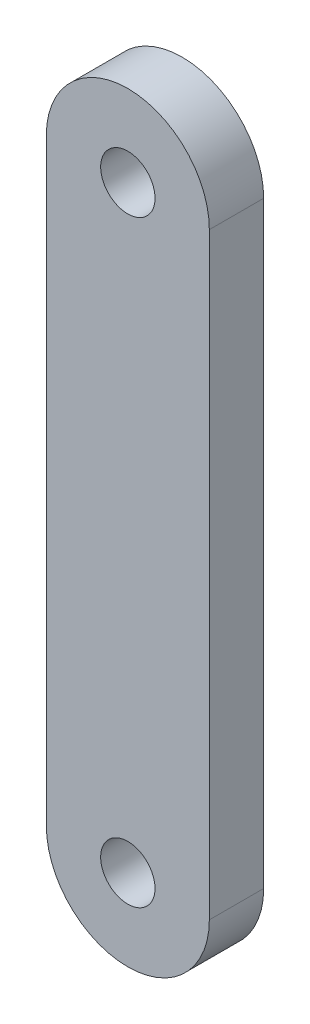
SolidWorks part; units mm, degrees
material "AISI 1045 钢，冷拔"
ref_plane "前视基准面" through (0, 0, 0) normal (0, 0, 1) x (1, 0, 0)
ref_plane "上视基准面" through (0, 0, 0) normal (0, 1, 0) x (1, 0, 0)
ref_plane "右视基准面" through (0, 0, 0) normal (1, 0, 0) x (0, 0, -1)
other "Configuration Table"
sketch "草图1" plane through (0, 0, 0) normal (0, 0, 1) x (1, 0, 0)
  line L0 (0, 0) -> (0, 110) construction
  line L1 (-15, 0) -> (-15, 110)
  line L2 (15, 0) -> (15, 110)
  arc A1 (-15, 0) -> (15, 0) centre (0, 0) ccw
  arc A2 (15, 110) -> (-15, 110) centre (0, 110) ccw
  circle A3 centre (0, 0) radius 5
  circle A4 centre (0, 110) radius 5
  point P3 (0, 55)
  dimension "D3" = 10
  dimension "D4" = 10
  dimension "D1" = 30
  dimension "D2" = 110
extrude "凸台-拉伸1" add sketch "草图1" along normal blind 10
